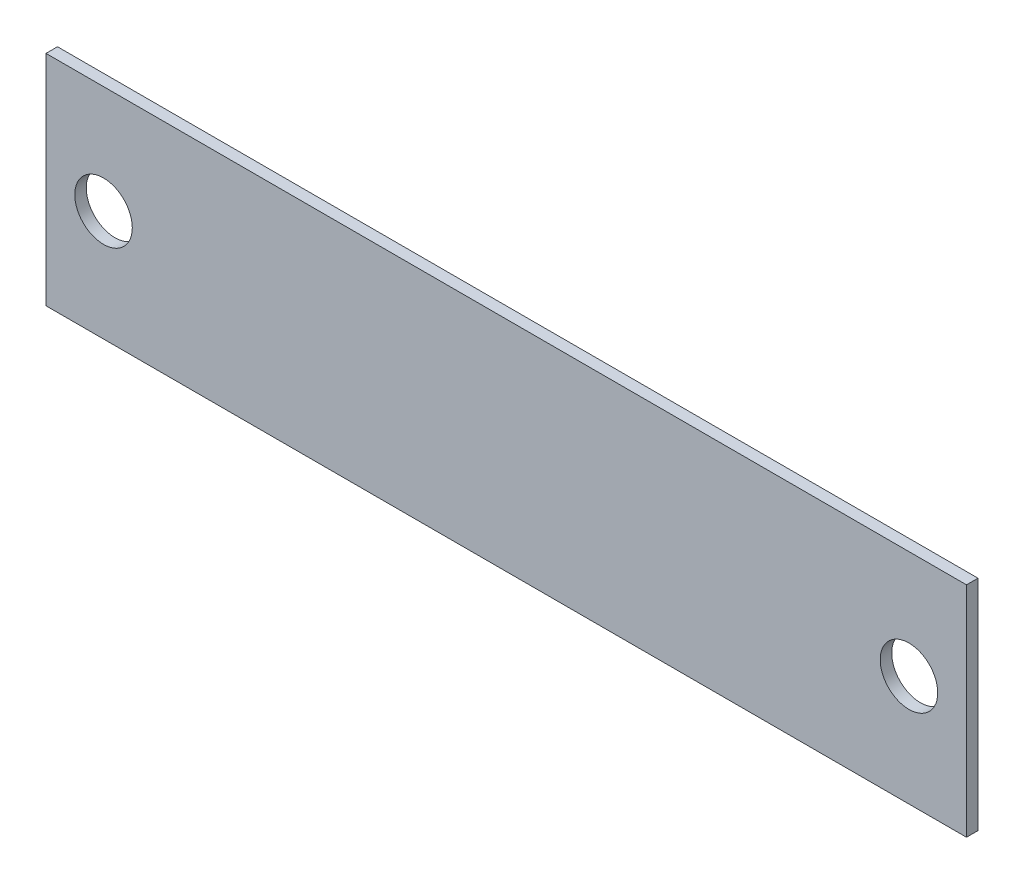
SolidWorks part; units mm, degrees
ref_plane "前视基准面" through (0, 0, 0) normal (0, 0, 1) x (1, 0, 0)
ref_plane "上视基准面" through (0, 0, 0) normal (0, 1, 0) x (1, 0, 0)
ref_plane "右视基准面" through (0, 0, 0) normal (1, 0, 0) x (0, 0, -1)
sketch "草图1" plane through (0, 0, 0) normal (0, 0, 1) x (1, 0, 0)
  line L1 (-40, 19) -> (40, 19)
  line L2 (-40, 19) -> (-40, 0)
  line L3 (-40, 0) -> (40, 0)
  line L4 (40, 19) -> (40, 0)
  dimension "D1" = 80
  dimension "D2" = 19
extrude "凸台-拉伸1" add sketch "草图1" along normal blind 1
hole_wizard "Ø5.0 (5) 直径孔1" positions "草图3" profile "草图2" hole size "Ø5.0" standard "GB" end condition through all
sketch "草图3" plane through (0, 0, 1) normal (0, 0, 1) x (1, 0, 0)
  line L0 (40, 0) -> (40, 19) construction
  line L1 (-40, 19) -> (-40, 0) construction
  point P0 (-35, 9.6219)
  point P2 (35, 9.6219)
  point P7 (-40, 9.5)
  dimension "D1" = 5
  dimension "D2" = 5
sketch "草图2" plane through (-35, 9.6219, 1) normal (1, 0, 0) x (0, -1, 0)
  line L0 (0, 0) -> (0, 1)
  line L1 (0, 1) -> (2.5, 1)
  line L2 (2.5, 1) -> (2.5, 0)
  line L5 (2.5, 0) -> (0, 0)
  line L11 (0, -6.35) -> (0, 107.95) construction
  dimension "通孔孔直径" = 5
  dimension "通孔孔深度" = 1
